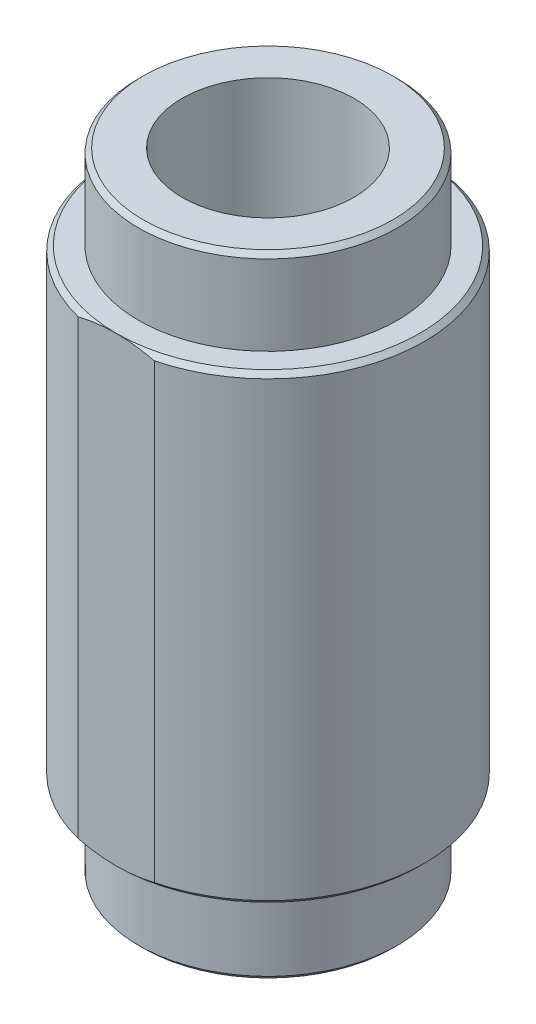
SolidWorks part; units mm, degrees
ref_plane "Front Plane" through (0, 0, 0) normal (0, 0, 1) x (1, 0, 0)
ref_plane "Top Plane" through (0, 0, 0) normal (0, 1, 0) x (1, 0, 0)
ref_plane "Right Plane" through (0, 0, 0) normal (1, 0, 0) x (0, 0, -1)
sketch "Sketch1" plane through (0, 0, 0) normal (0, 0, 1) x (1, 0, 0)
  line L0 (0, -26.6565) -> (0, 72.5099) construction
  line L1 (-66.5, 230) -> (-66.5, 38)
  line L2 (0, 0) -> (-66.5, 0) construction
  line L3 (-55, 266) -> (-55, 232)
  line L4 (-64.5, 36) -> (-55, 36)
  line L5 (-64.5, 232) -> (-55, 232)
  line L6 (-36.5, 268) -> (-36.5, 0)
  line L7 (-36.5, 0) -> (-53, 0)
  line L8 (-55, 36) -> (-55, 2)
  line L9 (-53, 268) -> (-36.5, 268)
  line L10 (-55, 266) -> (-53, 268)
  line L11 (-55, 2) -> (-53, 0)
  line L12 (-66.5, 38) -> (-64.5, 36)
  line L13 (-66.5, 230) -> (-64.5, 232)
  point P3 (-66.5, 232)
  point P6 (-55, 268)
  point P7 (-66.5, 36)
  point P15 (-55, 0)
  dimension "D1" = 133
  dimension "D2" = 110
  dimension "D3" = 36
  dimension "D4" = 73
  dimension "D5" = 268
  dimension "D6" = 36
revolve "Revolve1" add sketch "Sketch1" angle 360 about L0
sketch "Sketch2" plane through (0, 36, 0) normal (0, -1, 0) x (1, 0, 0)
  line L0 (0, 0) -> (-127.982, 0) construction
  line L1 (-16.1864, 64.5) -> (16.1864, 64.5)
  line L2 (-16.1864, -64.5) -> (16.1864, -64.5)
  circle A0 centre (0, 0) radius 66.5 construction
  arc A1 (-16.1864, -64.5) -> (16.1864, -64.5) centre (0, 0) ccw
  arc A2 (16.1864, 64.5) -> (-16.1864, 64.5) centre (0, 0) ccw
  dimension "D1" = 129
  dimension "D2" = 129
extrude "Cut-Extrude1" cut sketch "Sketch2" against normal through all
